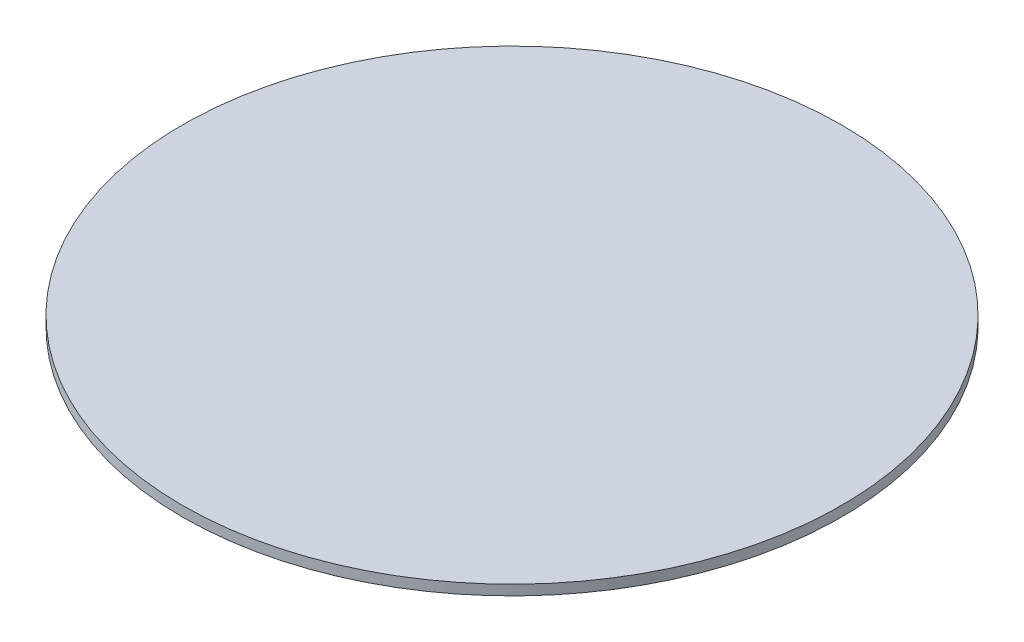
SolidWorks part; units mm, degrees
ref_plane "Front Plane" through (0, 0, 0) normal (0, 0, 1) x (1, 0, 0)
ref_plane "Top Plane" through (0, 0, 0) normal (0, 1, 0) x (1, 0, 0)
ref_plane "Right Plane" through (0, 0, 0) normal (1, 0, 0) x (0, 0, -1)
sketch "Sketch1" plane through (0, 0, 0) normal (0, 1, 0) x (1, 0, 0)
  circle A1 centre (0, 0) radius 32.5
  dimension "D1" = 65
extrude "Boss-Extrude1" add sketch "Sketch1" along normal blind 1
